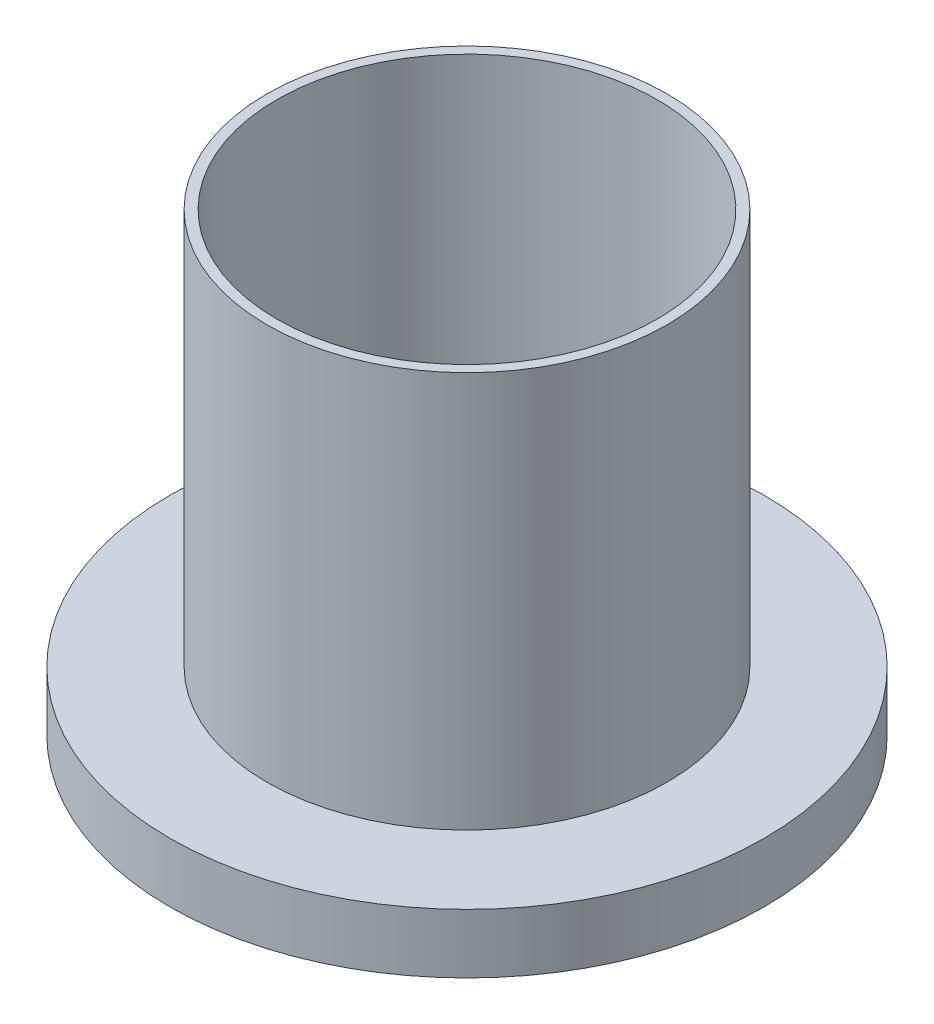
from build123d import *

# Parameters (mm, degrees)
SKETCH1_R           = 10.1
BOSS_EXTRUDE1_DEPTH = 20
BOSS_EXTRUDE2_START = 3
SKETCH2_R           = 15
BOSS_EXTRUDE2_DEPTH = 3
SKETCH4_R           = 9.6
CUT_EXTRUDE1_DEPTH  = 32.288975694


with BuildPart() as part:
    # Sketch1 → Boss-Extrude1 (new body)
    with BuildSketch(Plane(origin=(0, 0, 0), x_dir=(1, 0, 0), z_dir=(0, 1, 0))):
        with Locations(Location((0, 0, 0), (0, 0, 270))):
            Circle(SKETCH1_R)
    extrude(amount=BOSS_EXTRUDE1_DEPTH)

    # Sketch2 → Boss-Extrude2 (add)
    with BuildSketch(Plane.XZ.offset(BOSS_EXTRUDE2_START)):
        with Locations(Location((0, 0, 0), (0, 0, 270))):
            Circle(SKETCH2_R)
    extrude(amount=-BOSS_EXTRUDE2_DEPTH)

    # Sketch4 → Cut-Extrude1 (cut, through all)
    with BuildSketch(Plane(origin=(0, 20, 0), x_dir=(1, 0, 0), z_dir=(0, 1, 0))):
        with Locations(Location((0, 0, 0), (0, 0, 270))):
            Circle(SKETCH4_R)
    extrude(amount=-CUT_EXTRUDE1_DEPTH, mode=Mode.SUBTRACT)


solid = part.part
